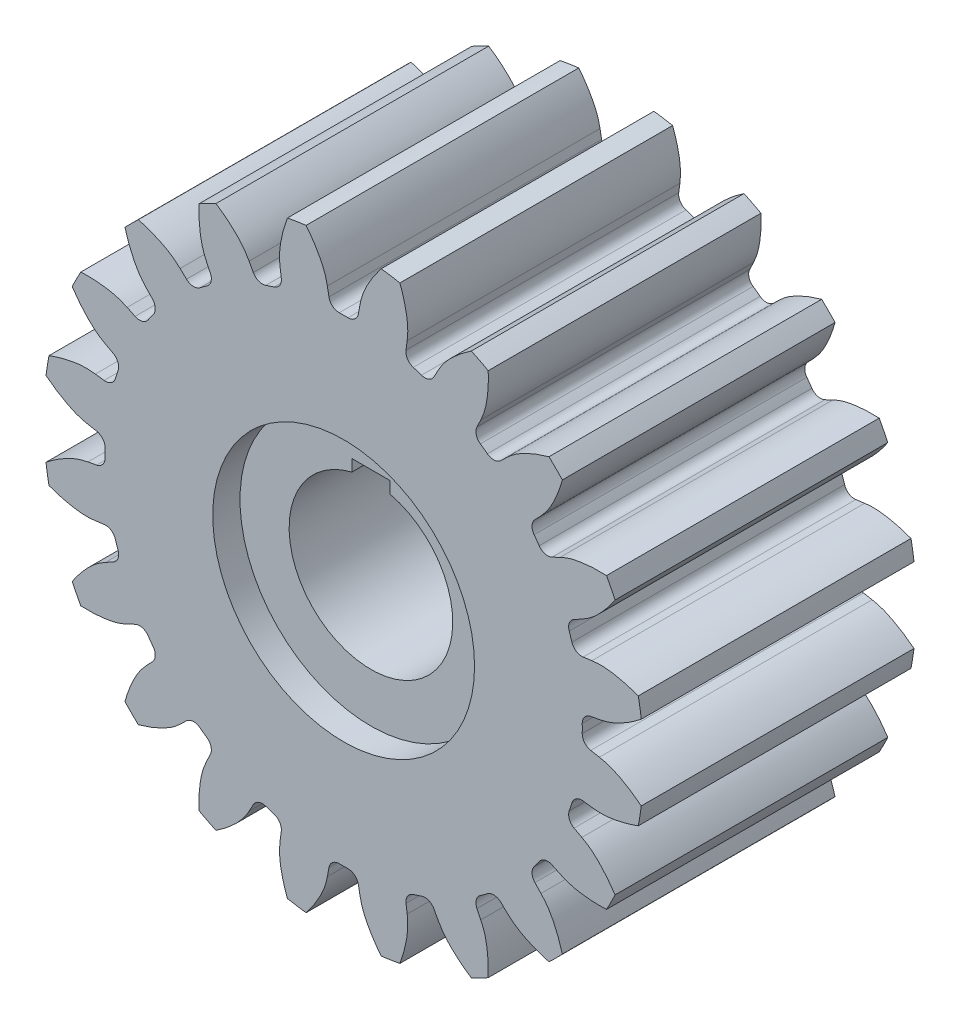
from build123d import *

# Parameters (mm, degrees)
BOSS_EXTRUDE1_DEPTH = 10
SKETCH6_R           = 9.6
SKETCH6_R_2         = 6
CUT_EXTRUDE2_DEPTH  = 2
CUT_EXTRUDE3_START  = -2
SKETCH7_R           = 9.6
SKETCH7_R_2         = 6
CUT_EXTRUDE3_DEPTH  = 2
SKETCH8_R           = 6
CUT_EXTRUDE4_DEPTH  = 37.780906003
SKETCH9_W           = 2.8
SKETCH9_H           = 1.7
CUT_EXTRUDE5_DEPTH  = 10


with BuildPart() as part:
    # Sketch1 → Boss-Extrude1 (new, symmetric)
    with BuildSketch(Plane.XY):
        with BuildLine():
            Line((17.567082995, 4.573202474), (18.207158907, 4.659211645))
            add(Edge.make_bspline(
                [(18.207158907, 4.659211645), (18.476950806, 4.695464497), (19.035752654, 4.728775845), (19.883742504, 4.619891848), (20.748748756, 4.422168203), (21.322633974, 4.234985171), (21.609620348, 4.126052401)],
                knots=[0, 0, 0, 0, 44.621092309, 91.187357158, 139.632096471, 189.949046908, 189.949046908, 189.949046908, 189.949046908], degree=3, weights=[1, 1, 1, 1, 1, 1, 1]))
            ThreePointArc((21.609620348, 4.126052401), (21.672084484, 3.784277225), (21.729143493, 3.441558231))
            ThreePointArc((21.729143493, 3.441558231), (21.780783144, 3.097980895), (21.826990558, 2.753630907))
            add(Edge.make_bspline(
                [(18.755812701, 1.195147926), (19.023602791, 1.244039696), (19.565348703, 1.385037989), (20.33818797, 1.750636099), (21.099757836, 2.205984092), (21.587712374, 2.56134602), (21.826990558, 2.753630907)],
                knots=[0, 0, 0, 0, 48.786983725, 99.700744187, 152.668356276, 207.6829719, 207.6829719, 207.6829719, 207.6829719], degree=3, weights=[1, 1, 1, 1, 1, 1, 1]))
            Line((18.755812701, 1.195147926), (18.120486038, 1.079153174))
            ThreePointArc((18.120486038, 1.079153174), (17.668922794, 0.812948127), (17.497115699, 0.317714028))
            ThreePointArc((17.497115699, 0.317714028), (17.49927891, 0.15886356), (17.5, 0))
            ThreePointArc((17.5, 0), (17.49927891, -0.15886356), (17.497115699, -0.317714028))
            ThreePointArc((17.497115699, -0.317714028), (17.668922794, -0.812948127), (18.120486038, -1.079153174))
            Line((18.120486038, -1.079153174), (18.755812701, -1.195147926))
            add(Edge.make_bspline(
                [(18.755812701, -1.195147926), (19.023602791, -1.244039696), (19.565348703, -1.385037989), (20.33818797, -1.750636099), (21.099757836, -2.205984092), (21.587712374, -2.56134602), (21.826990558, -2.753630907)],
                knots=[0, 0, 0, 0, 53.133990099, 108.584256495, 166.271376325, 226.187891319, 226.187891319, 226.187891319, 226.187891319], degree=3, weights=[1, 1, 1, 1, 1, 1, 1]))
            ThreePointArc((21.826990558, -2.753630907), (21.780783144, -3.097980895), (21.729143493, -3.441558231))
            ThreePointArc((21.729143493, -3.441558231), (21.672084484, -3.784277225), (21.609620348, -4.126052401))
            add(Edge.make_bspline(
                [(18.207158907, -4.659211645), (18.476950806, -4.695464497), (19.035752654, -4.728775845), (19.883742504, -4.619891848), (20.748748756, -4.422168203), (21.322633974, -4.234985171), (21.609620348, -4.126052401)],
                knots=[0, 0, 0, 0, 56.669331148, 115.809055132, 177.334464584, 241.237604986, 241.237604986, 241.237604986, 241.237604986], degree=3, weights=[1, 1, 1, 1, 1, 1, 1]))
            Line((18.207158907, -4.659211645), (17.567082995, -4.573202474))
            ThreePointArc((17.567082995, -4.573202474), (17.055358946, -4.686837802), (16.738924936, -5.104742107))
            ThreePointArc((16.738924936, -5.104742107), (16.691894778, -5.256486348), (16.643489035, -5.407797402))
            ThreePointArc((16.643489035, -5.407797402), (16.593711698, -5.558662797), (16.542566868, -5.709070101))
            ThreePointArc((16.542566868, -5.709070101), (16.552929373, -6.233157029), (16.900129654, -6.62587379))
            Line((16.900129654, -6.62587379), (17.468516867, -6.932518091))
            add(Edge.make_bspline(
                [(17.468516867, -6.932518091), (17.70809199, -7.061768617), (18.179752101, -7.363274655), (18.801789893, -7.949799587), (19.385375609, -8.618199294), (19.739635077, -9.106954816), (19.907782855, -9.363769636)],
                knots=[0, 0, 0, 0, 59.737720922, 122.079595359, 186.936329416, 254.299537876, 254.299537876, 254.299537876, 254.299537876], degree=3, weights=[1, 1, 1, 1, 1, 1, 1]))
            ThreePointArc((19.907782855, -9.363769636), (19.757426994, -9.67698706), (19.602143532, -9.987790994))
            ThreePointArc((19.602143532, -9.987790994), (19.441971196, -10.296103923), (19.276949935, -10.601848952))
            add(Edge.make_bspline(
                [(15.876261543, -10.057495117), (16.121646139, -10.17534391), (16.642804506, -10.379704152), (17.482937784, -10.538192592), (18.366707583, -10.617447863), (18.970347597, -10.616766506), (19.276949935, -10.601848952)],
                knots=[0, 0, 0, 0, 61.817188237, 126.329180452, 193.443574435, 263.15169308, 263.15169308, 263.15169308, 263.15169308], degree=3, weights=[1, 1, 1, 1, 1, 1, 1]))
            Line((15.876261543, -10.057495117), (15.294091471, -9.7779012))
            ThreePointArc((15.294091471, -9.7779012), (14.772297733, -9.727843392), (14.342211574, -10.027510517))
            ThreePointArc((14.342211574, -10.027510517), (14.250591685, -10.157294749), (14.157797402, -10.286241915))
            ThreePointArc((14.157797402, -10.286241915), (14.06383637, -10.414341389), (13.968716333, -10.541582614))
            ThreePointArc((13.968716333, -10.541582614), (13.816619893, -11.043221092), (14.02547083, -11.524007714))
            Line((14.02547083, -11.524007714), (14.471280893, -11.991285083))
            add(Edge.make_bspline(
                [(14.471280893, -11.991285083), (14.659189766, -12.188242422), (15.014594697, -12.620742695), (15.424941621, -13.370781302), (15.773417751, -14.186805103), (15.959304764, -14.761111423), (16.03986266, -15.057317352)],
                knots=[0, 0, 0, 0, 62.925887682, 128.594911008, 196.913010521, 267.871353491, 267.871353491, 267.871353491, 267.871353491], degree=3, weights=[1, 1, 1, 1, 1, 1, 1]))
            ThreePointArc((16.03986266, -15.057317352), (15.800076232, -15.308742308), (15.556349186, -15.556349186))
            ThreePointArc((15.556349186, -15.556349186), (15.308742308, -15.800076232), (15.057317352, -16.03986266))
            add(Edge.make_bspline(
                [(11.991285083, -14.471280893), (12.188242422, -14.659189766), (12.620742695, -15.014594697), (13.370781302, -15.424941621), (14.186805103, -15.773417751), (14.761111423, -15.959304764), (15.057317352, -16.03986266)],
                knots=[0, 0, 0, 0, 63.209035249, 129.173549427, 197.799059839, 269.076694008, 269.076694008, 269.076694008, 269.076694008], degree=3, weights=[1, 1, 1, 1, 1, 1, 1]))
            Line((11.991285083, -14.471280893), (11.524007714, -14.02547083))
            ThreePointArc((11.524007714, -14.02547083), (11.043221092, -13.816619893), (10.541582614, -13.968716333))
            ThreePointArc((10.541582614, -13.968716333), (10.414341389, -14.06383637), (10.286241915, -14.157797402))
            ThreePointArc((10.286241915, -14.157797402), (10.157294749, -14.250591685), (10.027510517, -14.342211574))
            ThreePointArc((10.027510517, -14.342211574), (9.727843392, -14.772297733), (9.7779012, -15.294091471))
            Line((9.7779012, -15.294091471), (10.057495117, -15.876261543))
            add(Edge.make_bspline(
                [(10.057495117, -15.876261543), (10.17534391, -16.121646139), (10.379704152, -16.642804506), (10.538192592, -17.482937784), (10.617447863, -18.366707583), (10.616766506, -18.970347597), (10.601848952, -19.276949935)],
                knots=[0, 0, 0, 0, 62.154254123, 127.018005977, 194.498349518, 264.586560325, 264.586560325, 264.586560325, 264.586560325], degree=3, weights=[1, 1, 1, 1, 1, 1, 1]))
            ThreePointArc((10.601848952, -19.276949935), (10.296103923, -19.441971196), (9.987790994, -19.602143532))
            ThreePointArc((9.987790994, -19.602143532), (9.67698706, -19.757426994), (9.363769636, -19.907782855))
            add(Edge.make_bspline(
                [(6.932518091, -17.468516867), (7.061768617, -17.70809199), (7.363274655, -18.179752101), (7.949799587, -18.801789893), (8.618199294, -19.385375609), (9.106954816, -19.739635077), (9.363769636, -19.907782855)],
                knots=[0, 0, 0, 0, 60.648107843, 123.940055804, 189.785189175, 258.17499495, 258.17499495, 258.17499495, 258.17499495], degree=3, weights=[1, 1, 1, 1, 1, 1, 1]))
            Line((6.932518091, -17.468516867), (6.62587379, -16.900129654))
            ThreePointArc((6.62587379, -16.900129654), (6.233157029, -16.552929373), (5.709070101, -16.542566868))
            ThreePointArc((5.709070101, -16.542566868), (5.558662797, -16.593711698), (5.407797402, -16.643489035))
            ThreePointArc((5.407797402, -16.643489035), (5.256486348, -16.691894778), (5.104742107, -16.738924936))
            ThreePointArc((5.104742107, -16.738924936), (4.686837802, -17.055358946), (4.573202474, -17.567082995))
            Line((4.573202474, -17.567082995), (4.659211645, -18.207158907))
            add(Edge.make_bspline(
                [(4.659211645, -18.207158907), (4.695464497, -18.476950806), (4.728775845, -19.035752654), (4.619891848, -19.883742504), (4.422168203, -20.748748756), (4.234985171, -21.322633974), (4.126052401, -21.609620348)],
                knots=[0, 0, 0, 0, 57.630300621, 117.772885735, 180.341611546, 245.328388652, 245.328388652, 245.328388652, 245.328388652], degree=3, weights=[1, 1, 1, 1, 1, 1, 1]))
            ThreePointArc((4.126052401, -21.609620348), (3.784277225, -21.672084484), (3.441558231, -21.729143493))
            ThreePointArc((3.441558231, -21.729143493), (3.097980895, -21.780783144), (2.753630907, -21.826990558))
            add(Edge.make_bspline(
                [(1.195147926, -18.755812701), (1.244039696, -19.023602791), (1.385037989, -19.565348703), (1.750636099, -20.33818797), (2.205984092, -21.099757836), (2.56134602, -21.587712374), (2.753630907, -21.826990558)],
                knots=[0, 0, 0, 0, 54.699372113, 111.783260407, 171.169902138, 232.851619308, 232.851619308, 232.851619308, 232.851619308], degree=3, weights=[1, 1, 1, 1, 1, 1, 1]))
            Line((1.195147926, -18.755812701), (1.079153174, -18.120486038))
            ThreePointArc((1.079153174, -18.120486038), (0.812948127, -17.668922794), (0.317714028, -17.497115699))
            ThreePointArc((0.317714028, -17.497115699), (0.15886356, -17.49927891), (0, -17.5))
            ThreePointArc((0, -17.5), (-0.15886356, -17.49927891), (-0.317714028, -17.497115699))
            ThreePointArc((-0.317714028, -17.497115699), (-0.812948127, -17.668922794), (-1.079153174, -18.120486038))
            Line((-1.079153174, -18.120486038), (-1.195147926, -18.755812701))
            add(Edge.make_bspline(
                [(-1.195147926, -18.755812701), (-1.244039696, -19.023602791), (-1.385037989, -19.565348703), (-1.750636099, -20.33818797), (-2.205984092, -21.099757836), (-2.56134602, -21.587712374), (-2.753630907, -21.826990558)],
                knots=[0, 0, 0, 0, 50.397015373, 102.990993781, 157.706603497, 214.536770431, 214.536770431, 214.536770431, 214.536770431], degree=3, weights=[1, 1, 1, 1, 1, 1, 1]))
            ThreePointArc((-2.753630907, -21.826990558), (-3.097980895, -21.780783144), (-3.441558231, -21.729143493))
            ThreePointArc((-3.441558231, -21.729143493), (-3.784277225, -21.672084484), (-4.126052401, -21.609620348))
            add(Edge.make_bspline(
                [(-4.659211645, -18.207158907), (-4.695464497, -18.476950806), (-4.728775845, -19.035752654), (-4.619891848, -19.883742504), (-4.422168203, -20.748748756), (-4.234985171, -21.322633974), (-4.126052401, -21.609620348)],
                knots=[0, 0, 0, 0, 46.92324161, 95.892013626, 146.836176797, 199.74914464, 199.74914464, 199.74914464, 199.74914464], degree=3, weights=[1, 1, 1, 1, 1, 1, 1]))
            Line((-4.659211645, -18.207158907), (-4.573202474, -17.567082995))
            ThreePointArc((-4.573202474, -17.567082995), (-4.686837802, -17.055358946), (-5.104742107, -16.738924936))
            ThreePointArc((-5.104742107, -16.738924936), (-5.256486348, -16.691894778), (-5.407797402, -16.643489035))
            ThreePointArc((-5.407797402, -16.643489035), (-5.558662797, -16.593711698), (-5.709070101, -16.542566868))
            ThreePointArc((-5.709070101, -16.542566868), (-6.233157029, -16.552929373), (-6.62587379, -16.900129654))
            Line((-6.62587379, -16.900129654), (-6.932518091, -17.468516867))
            add(Edge.make_bspline(
                [(-6.932518091, -17.468516867), (-7.061768617, -17.70809199), (-7.363274655, -18.179752101), (-7.949799587, -18.801789893), (-8.618199294, -19.385375609), (-9.106954816, -19.739635077), (-9.363769636, -19.907782855)],
                knots=[0, 0, 0, 0, 42.798548369, 87.462818905, 133.928837808, 182.190597565, 182.190597565, 182.190597565, 182.190597565], degree=3, weights=[1, 1, 1, 1, 1, 1, 1]))
            ThreePointArc((-9.363769636, -19.907782855), (-9.67698706, -19.757426994), (-9.987790994, -19.602143532))
            ThreePointArc((-9.987790994, -19.602143532), (-10.296103923, -19.441971196), (-10.601848952, -19.276949935))
            add(Edge.make_bspline(
                [(-10.057495117, -15.876261543), (-10.17534391, -16.121646139), (-10.379704152, -16.642804506), (-10.538192592, -17.482937784), (-10.617447863, -18.366707583), (-10.616766506, -18.970347597), (-10.601848952, -19.276949935)],
                knots=[0, 0, 0, 0, 40.519446674, 82.805262367, 126.79688, 172.488611973, 172.488611973, 172.488611973, 172.488611973], degree=3, weights=[1, 1, 1, 1, 1, 1, 1]))
            Line((-10.057495117, -15.876261543), (-9.7779012, -15.294091471))
            ThreePointArc((-9.7779012, -15.294091471), (-9.727843392, -14.772297733), (-10.027510517, -14.342211574))
            ThreePointArc((-10.027510517, -14.342211574), (-10.157294749, -14.250591685), (-10.286241915, -14.157797402))
            ThreePointArc((-10.286241915, -14.157797402), (-10.414341389, -14.06383637), (-10.541582614, -13.968716333))
            ThreePointArc((-10.541582614, -13.968716333), (-11.043221092, -13.816619893), (-11.524007714, -14.02547083))
            Line((-11.524007714, -14.02547083), (-11.991285083, -14.471280893))
            add(Edge.make_bspline(
                [(-11.991285083, -14.471280893), (-12.188242422, -14.659189766), (-12.620742695, -15.014594697), (-13.370781302, -15.424941621), (-14.186805103, -15.773417751), (-14.761111423, -15.959304764), (-15.057317352, -16.03986266)],
                knots=[0, 0, 0, 0, 38.79262688, 79.276345319, 121.393169431, 165.137654003, 165.137654003, 165.137654003, 165.137654003], degree=3, weights=[1, 1, 1, 1, 1, 1, 1]))
            ThreePointArc((-15.057317352, -16.03986266), (-15.308742308, -15.800076232), (-15.556349186, -15.556349186))
            ThreePointArc((-15.556349186, -15.556349186), (-15.800076232, -15.308742308), (-16.03986266, -15.057317352))
            add(Edge.make_bspline(
                [(-14.471280893, -11.991285083), (-14.659189766, -12.188242422), (-15.014594697, -12.620742695), (-15.424941621, -13.370781302), (-15.773417751, -14.186805103), (-15.959304764, -14.761111423), (-16.03986266, -15.057317352)],
                knots=[0, 0, 0, 0, 39.262662903, 80.2369077, 122.864045913, 167.138566349, 167.138566349, 167.138566349, 167.138566349], degree=3, weights=[1, 1, 1, 1, 1, 1, 1]))
            Line((-14.471280893, -11.991285083), (-14.02547083, -11.524007714))
            ThreePointArc((-14.02547083, -11.524007714), (-13.816619893, -11.043221092), (-13.968716333, -10.541582614))
            ThreePointArc((-13.968716333, -10.541582614), (-14.06383637, -10.414341389), (-14.157797402, -10.286241915))
            ThreePointArc((-14.157797402, -10.286241915), (-14.250591685, -10.157294749), (-14.342211574, -10.027510517))
            ThreePointArc((-14.342211574, -10.027510517), (-14.772297733, -9.727843392), (-15.294091471, -9.7779012))
            Line((-15.294091471, -9.7779012), (-15.876261543, -10.057495117))
            add(Edge.make_bspline(
                [(-15.876261543, -10.057495117), (-16.121646139, -10.17534391), (-16.642804506, -10.379704152), (-17.482937784, -10.538192592), (-18.366707583, -10.617447863), (-18.970347597, -10.616766506), (-19.276949935, -10.601848952)],
                knots=[0, 0, 0, 0, 40.908743076, 83.600825814, 128.01509923, 174.145821077, 174.145821077, 174.145821077, 174.145821077], degree=3, weights=[1, 1, 1, 1, 1, 1, 1]))
            ThreePointArc((-19.276949935, -10.601848952), (-19.441971196, -10.296103923), (-19.602143532, -9.987790994))
            ThreePointArc((-19.602143532, -9.987790994), (-19.757426994, -9.67698706), (-19.907782855, -9.363769636))
            add(Edge.make_bspline(
                [(-17.468516867, -6.932518091), (-17.70809199, -7.061768617), (-18.179752101, -7.363274655), (-18.801789893, -7.949799587), (-19.385375609, -8.618199294), (-19.739635077, -9.106954816), (-19.907782855, -9.363769636)],
                knots=[0, 0, 0, 0, 44.029427389, 89.9782348, 137.780608556, 187.430368369, 187.430368369, 187.430368369, 187.430368369], degree=3, weights=[1, 1, 1, 1, 1, 1, 1]))
            Line((-17.468516867, -6.932518091), (-16.900129654, -6.62587379))
            ThreePointArc((-16.900129654, -6.62587379), (-16.552929373, -6.233157029), (-16.542566868, -5.709070101))
            ThreePointArc((-16.542566868, -5.709070101), (-16.593711698, -5.558662797), (-16.643489035, -5.407797402))
            ThreePointArc((-16.643489035, -5.407797402), (-16.691894778, -5.256486348), (-16.738924936, -5.104742107))
            ThreePointArc((-16.738924936, -5.104742107), (-17.055358946, -4.686837802), (-17.567082995, -4.573202474))
            Line((-17.567082995, -4.573202474), (-18.207158907, -4.659211645))
            add(Edge.make_bspline(
                [(-18.207158907, -4.659211645), (-18.476950806, -4.695464497), (-19.035752654, -4.728775845), (-19.883742504, -4.619891848), (-20.748748756, -4.422168203), (-21.322633974, -4.234985171), (-21.609620348, -4.126052401)],
                knots=[0, 0, 0, 0, 48.099346598, 98.295493687, 150.516544013, 204.755746006, 204.755746006, 204.755746006, 204.755746006], degree=3, weights=[1, 1, 1, 1, 1, 1, 1]))
            ThreePointArc((-21.609620348, -4.126052401), (-21.672084484, -3.784277225), (-21.729143493, -3.441558231))
            ThreePointArc((-21.729143493, -3.441558231), (-21.780783144, -3.097980895), (-21.826990558, -2.753630907))
            add(Edge.make_bspline(
                [(-18.755812701, -1.195147926), (-19.023602791, -1.244039696), (-19.565348703, -1.385037989), (-20.33818797, -1.750636099), (-21.099757836, -2.205984092), (-21.587712374, -2.56134602), (-21.826990558, -2.753630907)],
                knots=[0, 0, 0, 0, 52.173738756, 106.621893459, 163.266476597, 222.100164687, 222.100164687, 222.100164687, 222.100164687], degree=3, weights=[1, 1, 1, 1, 1, 1, 1]))
            Line((-18.755812701, -1.195147926), (-18.120486038, -1.079153174))
            ThreePointArc((-18.120486038, -1.079153174), (-17.668922794, -0.812948127), (-17.497115699, -0.317714028))
            ThreePointArc((-17.497115699, -0.317714028), (-17.49927891, -0.15886356), (-17.5, 0))
            ThreePointArc((-17.5, 0), (-17.49927891, 0.15886356), (-17.497115699, 0.317714028))
            ThreePointArc((-17.497115699, 0.317714028), (-17.668922794, 0.812948127), (-18.120486038, 1.079153174))
            Line((-18.120486038, 1.079153174), (-18.755812701, 1.195147926))
            add(Edge.make_bspline(
                [(-18.755812701, 1.195147926), (-19.023602791, 1.244039696), (-19.565348703, 1.385037989), (-20.33818797, 1.750636099), (-21.099757836, 2.205984092), (-21.587712374, 2.56134602), (-21.826990558, 2.753630907)],
                knots=[0, 0, 0, 0, 56.345383077, 115.147037085, 176.32073888, 239.858579417, 239.858579417, 239.858579417, 239.858579417], degree=3, weights=[1, 1, 1, 1, 1, 1, 1]))
            ThreePointArc((-21.826990558, 2.753630907), (-21.780783144, 3.097980895), (-21.729143493, 3.441558231))
            ThreePointArc((-21.729143493, 3.441558231), (-21.672084484, 3.784277225), (-21.609620348, 4.126052401))
            add(Edge.make_bspline(
                [(-18.207158907, 4.659211645), (-18.476950806, 4.695464497), (-19.035752654, 4.728775845), (-19.883742504, 4.619891848), (-20.748748756, 4.422168203), (-21.322633974, 4.234985171), (-21.609620348, 4.126052401)],
                knots=[0, 0, 0, 0, 59.722479696, 122.048448495, 186.888635283, 254.234656983, 254.234656983, 254.234656983, 254.234656983], degree=3, weights=[1, 1, 1, 1, 1, 1, 1]))
            Line((-18.207158907, 4.659211645), (-17.567082995, 4.573202474))
            ThreePointArc((-17.567082995, 4.573202474), (-17.055358946, 4.686837802), (-16.738924936, 5.104742107))
            ThreePointArc((-16.738924936, 5.104742107), (-16.691894778, 5.256486348), (-16.643489035, 5.407797402))
            ThreePointArc((-16.643489035, 5.407797402), (-16.593711698, 5.558662797), (-16.542566868, 5.709070101))
            ThreePointArc((-16.542566868, 5.709070101), (-16.552929373, 6.233157029), (-16.900129654, 6.62587379))
            Line((-16.900129654, 6.62587379), (-17.468516867, 6.932518091))
            add(Edge.make_bspline(
                [(-17.468516867, 6.932518091), (-17.70809199, 7.061768617), (-18.179752101, 7.363274655), (-18.801789893, 7.949799587), (-19.385375609, 8.618199294), (-19.739635077, 9.106954816), (-19.907782855, 9.363769636)],
                knots=[0, 0, 0, 0, 62.538800152, 127.803861596, 195.70170348, 266.223547407, 266.223547407, 266.223547407, 266.223547407], degree=3, weights=[1, 1, 1, 1, 1, 1, 1]))
            ThreePointArc((-19.907782855, 9.363769636), (-19.757426994, 9.67698706), (-19.602143532, 9.987790994))
            ThreePointArc((-19.602143532, 9.987790994), (-19.441971196, 10.296103923), (-19.276949935, 10.601848952))
            add(Edge.make_bspline(
                [(-15.876261543, 10.057495117), (-16.121646139, 10.17534391), (-16.642804506, 10.379704152), (-17.482937784, 10.538192592), (-18.366707583, 10.617447863), (-18.970347597, 10.616766506), (-19.276949935, 10.601848952)],
                knots=[0, 0, 0, 0, 64.400604659, 131.608632473, 201.527819629, 274.149126395, 274.149126395, 274.149126395, 274.149126395], degree=3, weights=[1, 1, 1, 1, 1, 1, 1]))
            Line((-15.876261543, 10.057495117), (-15.294091471, 9.7779012))
            ThreePointArc((-15.294091471, 9.7779012), (-14.772297733, 9.727843392), (-14.342211574, 10.027510517))
            ThreePointArc((-14.342211574, 10.027510517), (-14.250591685, 10.157294749), (-14.157797402, 10.286241915))
            ThreePointArc((-14.157797402, 10.286241915), (-14.06383637, 10.414341389), (-13.968716333, 10.541582614))
            ThreePointArc((-13.968716333, 10.541582614), (-13.816619893, 11.043221092), (-14.02547083, 11.524007714))
            Line((-14.02547083, 11.524007714), (-14.471280893, 11.991285083))
            add(Edge.make_bspline(
                [(-14.471280893, 11.991285083), (-14.659189766, 12.188242422), (-15.014594697, 12.620742695), (-15.424941621, 13.370781302), (-15.773417751, 14.186805103), (-15.959304764, 14.761111423), (-16.03986266, 15.057317352)],
                knots=[0, 0, 0, 0, 65.184441139, 133.210475309, 203.980667045, 277.485866591, 277.485866591, 277.485866591, 277.485866591], degree=3, weights=[1, 1, 1, 1, 1, 1, 1]))
            ThreePointArc((-16.03986266, 15.057317352), (-15.800076232, 15.308742308), (-15.556349186, 15.556349186))
            ThreePointArc((-15.556349186, 15.556349186), (-15.308742308, 15.800076232), (-15.057317352, 16.03986266))
            add(Edge.make_bspline(
                [(-11.991285083, 14.471280893), (-12.188242422, 14.659189766), (-12.620742695, 15.014594697), (-13.370781302, 15.424941621), (-14.186805103, 15.773417751), (-14.761111423, 15.959304764), (-15.057317352, 16.03986266)],
                knots=[0, 0, 0, 0, 65.189629174, 133.221077543, 203.996901886, 277.507951716, 277.507951716, 277.507951716, 277.507951716], degree=3, weights=[1, 1, 1, 1, 1, 1, 1]))
            Line((-11.991285083, 14.471280893), (-11.524007714, 14.02547083))
            ThreePointArc((-11.524007714, 14.02547083), (-11.043221092, 13.816619893), (-10.541582614, 13.968716333))
            ThreePointArc((-10.541582614, 13.968716333), (-10.414341389, 14.06383637), (-10.286241915, 14.157797402))
            ThreePointArc((-10.286241915, 14.157797402), (-10.157294749, 14.250591685), (-10.027510517, 14.342211574))
            ThreePointArc((-10.027510517, 14.342211574), (-9.727843392, 14.772297733), (-9.7779012, 15.294091471))
            Line((-9.7779012, 15.294091471), (-10.057495117, 15.876261543))
            add(Edge.make_bspline(
                [(-10.057495117, 15.876261543), (-10.17534391, 16.121646139), (-10.379704152, 16.642804506), (-10.538192592, 17.482937784), (-10.617447863, 18.366707583), (-10.616766506, 18.970347597), (-10.601848952, 19.276949935)],
                knots=[0, 0, 0, 0, 63.731799596, 130.241867049, 199.434938254, 271.302067355, 271.302067355, 271.302067355, 271.302067355], degree=3, weights=[1, 1, 1, 1, 1, 1, 1]))
            ThreePointArc((-10.601848952, 19.276949935), (-10.296103923, 19.441971196), (-9.987790994, 19.602143532))
            ThreePointArc((-9.987790994, 19.602143532), (-9.67698706, 19.757426994), (-9.363769636, 19.907782855))
            add(Edge.make_bspline(
                [(-6.932518091, 17.468516867), (-7.061768617, 17.70809199), (-7.363274655, 18.179752101), (-7.949799587, 18.801789893), (-8.618199294, 19.385375609), (-9.106954816, 19.739635077), (-9.363769636, 19.907782855)],
                knots=[0, 0, 0, 0, 61.882295751, 126.462233719, 193.647314374, 263.428851471, 263.428851471, 263.428851471, 263.428851471], degree=3, weights=[1, 1, 1, 1, 1, 1, 1]))
            Line((-6.932518091, 17.468516867), (-6.62587379, 16.900129654))
            ThreePointArc((-6.62587379, 16.900129654), (-6.233157029, 16.552929373), (-5.709070101, 16.542566868))
            ThreePointArc((-5.709070101, 16.542566868), (-5.558662797, 16.593711698), (-5.407797402, 16.643489035))
            ThreePointArc((-5.407797402, 16.643489035), (-5.256486348, 16.691894778), (-5.104742107, 16.738924936))
            ThreePointArc((-5.104742107, 16.738924936), (-4.686837802, 17.055358946), (-4.573202474, 17.567082995))
            Line((-4.573202474, 17.567082995), (-4.659211645, 18.207158907))
            add(Edge.make_bspline(
                [(-4.659211645, 18.207158907), (-4.695464497, 18.476950806), (-4.728775845, 19.035752654), (-4.619891848, 19.883742504), (-4.422168203, 20.748748756), (-4.234985171, 21.322633974), (-4.126052401, 21.609620348)],
                knots=[0, 0, 0, 0, 58.365766856, 119.275879471, 182.643094701, 248.459219906, 248.459219906, 248.459219906, 248.459219906], degree=3, weights=[1, 1, 1, 1, 1, 1, 1]))
            ThreePointArc((-4.126052401, 21.609620348), (-3.784277225, 21.672084484), (-3.441558231, 21.729143493))
            ThreePointArc((-3.441558231, 21.729143493), (-3.097980895, 21.780783144), (-2.753630907, 21.826990558))
            add(Edge.make_bspline(
                [(-1.195147926, 18.755812701), (-1.244039696, 19.023602791), (-1.385037989, 19.565348703), (-1.750636099, 20.33818797), (-2.205984092, 21.099757836), (-2.56134602, 21.587712374), (-2.753630907, 21.826990558)],
                knots=[0, 0, 0, 0, 55.007403621, 112.412751477, 172.133820389, 234.162889121, 234.162889121, 234.162889121, 234.162889121], degree=3, weights=[1, 1, 1, 1, 1, 1, 1]))
            Line((-1.195147926, 18.755812701), (-1.079153174, 18.120486038))
            ThreePointArc((-1.079153174, 18.120486038), (-0.812948127, 17.668922794), (-0.317714028, 17.497115699))
            ThreePointArc((-0.317714028, 17.497115699), (-0.15886356, 17.49927891), (0, 17.5))
            ThreePointArc((0, 17.5), (0.15886356, 17.49927891), (0.317714028, 17.497115699))
            ThreePointArc((0.317714028, 17.497115699), (0.812948127, 17.668922794), (1.079153174, 18.120486038))
            Line((1.079153174, 18.120486038), (1.195147926, 18.755812701))
            add(Edge.make_bspline(
                [(1.195147926, 18.755812701), (1.244039696, 19.023602791), (1.385037989, 19.565348703), (1.750636099, 20.33818797), (2.205984092, 21.099757836), (2.56134602, 21.587712374), (2.753630907, 21.826990558)],
                knots=[0, 0, 0, 0, 50.061410911, 102.305154813, 156.656401627, 213.108124373, 213.108124373, 213.108124373, 213.108124373], degree=3, weights=[1, 1, 1, 1, 1, 1, 1]))
            ThreePointArc((2.753630907, 21.826990558), (3.097980895, 21.780783144), (3.441558231, 21.729143493))
            ThreePointArc((3.441558231, 21.729143493), (3.784277225, 21.672084484), (4.126052401, 21.609620348))
            add(Edge.make_bspline(
                [(4.659211645, 18.207158907), (4.695464497, 18.476950806), (4.728775845, 19.035752654), (4.619891848, 19.883742504), (4.422168203, 20.748748756), (4.234985171, 21.322633974), (4.126052401, 21.609620348)],
                knots=[0, 0, 0, 0, 46.029665803, 94.065908256, 144.039923796, 195.945251367, 195.945251367, 195.945251367, 195.945251367], degree=3, weights=[1, 1, 1, 1, 1, 1, 1]))
            Line((4.659211645, 18.207158907), (4.573202474, 17.567082995))
            ThreePointArc((4.573202474, 17.567082995), (4.686837802, 17.055358946), (5.104742107, 16.738924936))
            ThreePointArc((5.104742107, 16.738924936), (5.256486348, 16.691894778), (5.407797402, 16.643489035))
            ThreePointArc((5.407797402, 16.643489035), (5.558662797, 16.593711698), (5.709070101, 16.542566868))
            ThreePointArc((5.709070101, 16.542566868), (6.233157029, 16.552929373), (6.62587379, 16.900129654))
            Line((6.62587379, 16.900129654), (6.932518091, 17.468516867))
            add(Edge.make_bspline(
                [(6.932518091, 17.468516867), (7.061768617, 17.70809199), (7.363274655, 18.179752101), (7.949799587, 18.801789893), (8.618199294, 19.385375609), (9.106954816, 19.739635077), (9.363769636, 19.907782855)],
                knots=[0, 0, 0, 0, 41.056953981, 83.903708599, 128.478893331, 174.776745124, 174.776745124, 174.776745124, 174.776745124], degree=3, weights=[1, 1, 1, 1, 1, 1, 1]))
            ThreePointArc((9.363769636, 19.907782855), (9.67698706, 19.757426994), (9.987790994, 19.602143532))
            ThreePointArc((9.987790994, 19.602143532), (10.296103923, 19.441971196), (10.601848952, 19.276949935))
            add(Edge.make_bspline(
                [(10.057495117, 15.876261543), (10.17534391, 16.121646139), (10.379704152, 16.642804506), (10.538192592, 17.482937784), (10.617447863, 18.366707583), (10.616766506, 18.970347597), (10.601848952, 19.276949935)],
                knots=[0, 0, 0, 0, 38.160336318, 77.984200679, 119.414552322, 162.446034786, 162.446034786, 162.446034786, 162.446034786], degree=3, weights=[1, 1, 1, 1, 1, 1, 1]))
            Line((10.057495117, 15.876261543), (9.7779012, 15.294091471))
            ThreePointArc((9.7779012, 15.294091471), (9.727843392, 14.772297733), (10.027510517, 14.342211574))
            ThreePointArc((10.027510517, 14.342211574), (10.157294749, 14.250591685), (10.286241915, 14.157797402))
            ThreePointArc((10.286241915, 14.157797402), (10.414341389, 14.06383637), (10.541582614, 13.968716333))
            ThreePointArc((10.541582614, 13.968716333), (11.043221092, 13.816619893), (11.524007714, 14.02547083))
            Line((11.524007714, 14.02547083), (11.991285083, 14.471280893))
            add(Edge.make_bspline(
                [(11.991285083, 14.471280893), (12.188242422, 14.659189766), (12.620742695, 15.014594697), (13.370781302, 15.424941621), (14.186805103, 15.773417751), (14.761111423, 15.959304764), (15.057317352, 16.03986266)],
                knots=[0, 0, 0, 0, 35.757785364, 73.074364083, 111.896286647, 152.218533836, 152.218533836, 152.218533836, 152.218533836], degree=3, weights=[1, 1, 1, 1, 1, 1, 1]))
            ThreePointArc((15.057317352, 16.03986266), (15.308742308, 15.800076232), (15.556349186, 15.556349186))
            ThreePointArc((15.556349186, 15.556349186), (15.800076232, 15.308742308), (16.03986266, 15.057317352))
            add(Edge.make_bspline(
                [(14.471280893, 11.991285083), (14.659189766, 12.188242422), (15.014594697, 12.620742695), (15.424941621, 13.370781302), (15.773417751, 14.186805103), (15.959304764, 14.761111423), (16.03986266, 15.057317352)],
                knots=[0, 0, 0, 0, 35.955531437, 73.478476596, 112.515090385, 153.060325825, 153.060325825, 153.060325825, 153.060325825], degree=3, weights=[1, 1, 1, 1, 1, 1, 1]))
            Line((14.471280893, 11.991285083), (14.02547083, 11.524007714))
            ThreePointArc((14.02547083, 11.524007714), (13.816619893, 11.043221092), (13.968716333, 10.541582614))
            ThreePointArc((13.968716333, 10.541582614), (14.06383637, 10.414341389), (14.157797402, 10.286241915))
            ThreePointArc((14.157797402, 10.286241915), (14.250591685, 10.157294749), (14.342211574, 10.027510517))
            ThreePointArc((14.342211574, 10.027510517), (14.772297733, 9.727843392), (15.294091471, 9.7779012))
            Line((15.294091471, 9.7779012), (15.876261543, 10.057495117))
            add(Edge.make_bspline(
                [(15.876261543, 10.057495117), (16.121646139, 10.17534391), (16.642804506, 10.379704152), (17.482937784, 10.538192592), (18.366707583, 10.617447863), (18.970347597, 10.616766506), (19.276949935, 10.601848952)],
                knots=[0, 0, 0, 0, 37.395678309, 76.421550833, 117.021719797, 159.190936073, 159.190936073, 159.190936073, 159.190936073], degree=3, weights=[1, 1, 1, 1, 1, 1, 1]))
            ThreePointArc((19.276949935, 10.601848952), (19.441971196, 10.296103923), (19.602143532, 9.987790994))
            ThreePointArc((19.602143532, 9.987790994), (19.757426994, 9.67698706), (19.907782855, 9.363769636))
            add(Edge.make_bspline(
                [(17.468516867, 6.932518091), (17.70809199, 7.061768617), (18.179752101, 7.363274655), (18.801789893, 7.949799587), (19.385375609, 8.618199294), (19.739635077, 9.106954816), (19.907782855, 9.363769636)],
                knots=[0, 0, 0, 0, 40.494060185, 82.753382711, 126.717438449, 172.38054336, 172.38054336, 172.38054336, 172.38054336], degree=3, weights=[1, 1, 1, 1, 1, 1, 1]))
            Line((17.468516867, 6.932518091), (16.900129654, 6.62587379))
            ThreePointArc((16.900129654, 6.62587379), (16.552929373, 6.233157029), (16.542566868, 5.709070101))
            ThreePointArc((16.542566868, 5.709070101), (16.593711698, 5.558662797), (16.643489035, 5.407797402))
            ThreePointArc((16.643489035, 5.407797402), (16.691894778, 5.256486348), (16.738924936, 5.104742107))
            ThreePointArc((16.738924936, 5.104742107), (17.055358946, 4.686837802), (17.567082995, 4.573202474))
        make_face()
    extrude(amount=BOSS_EXTRUDE1_DEPTH, both=True)

    # Sketch6 → Cut-Extrude2 (cut)
    with BuildSketch(Plane(origin=(0, 0, -10), x_dir=(-1, 0, 0), z_dir=(0, 0, -1))):
        Circle(SKETCH6_R)
        Circle(SKETCH6_R_2, mode=Mode.SUBTRACT)
    extrude(amount=-CUT_EXTRUDE2_DEPTH, mode=Mode.SUBTRACT)

    # Sketch7 → Cut-Extrude3 (cut)
    with BuildSketch(Plane.XY.offset(10).offset(CUT_EXTRUDE3_START)):
        with Locations(Location((0, 0, 0), (0, 0, 180))):
            Circle(SKETCH7_R)
        with Locations(Location((0, 0, 0), (0, 0, 180))):
            Circle(SKETCH7_R_2, mode=Mode.SUBTRACT)
    extrude(amount=CUT_EXTRUDE3_DEPTH, mode=Mode.SUBTRACT)

    # Sketch8 → Cut-Extrude4 (cut, through all)
    with BuildSketch(Plane.XY.offset(10)):
        Circle(SKETCH8_R)
    extrude(amount=-CUT_EXTRUDE4_DEPTH, mode=Mode.SUBTRACT)

    # Sketch9 → Cut-Extrude5 (cut, symmetric)
    with BuildSketch(Plane.XY):
        with Locations((0, 5.85)):
            Rectangle(SKETCH9_W, SKETCH9_H)
    extrude(amount=CUT_EXTRUDE5_DEPTH, both=True, mode=Mode.SUBTRACT)


solid = part.part
